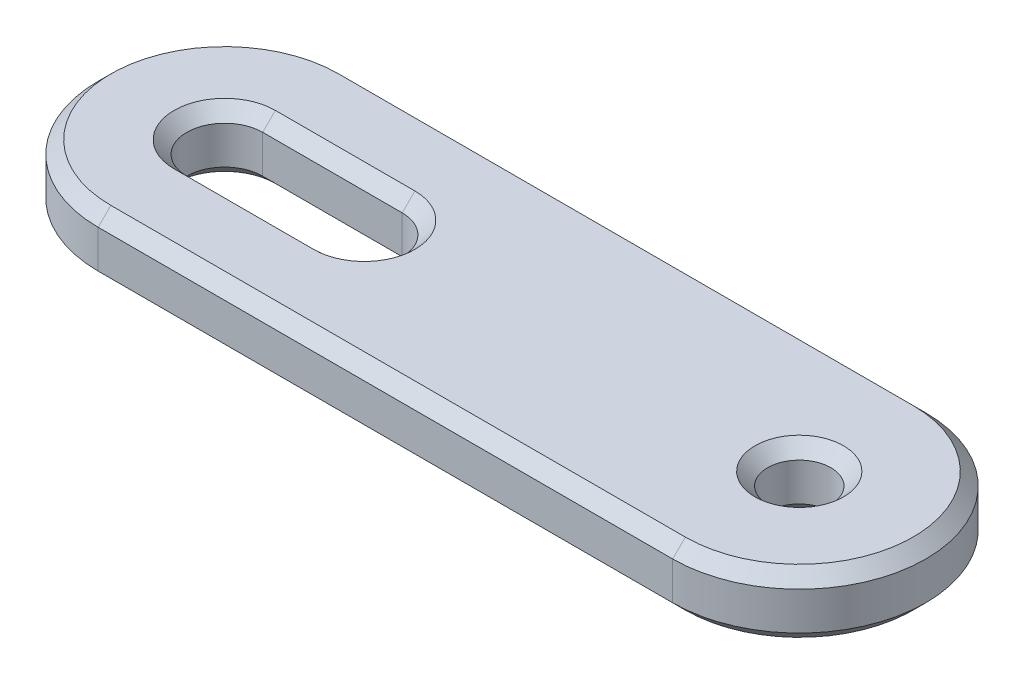
from build123d import *

# Parameters (mm, degrees)
SKETCH1_R           = 2.5
BOSS_EXTRUDE1_DEPTH = 5
CHAMFER1_SIZE       = 1


with BuildPart() as part:
    # Sketch1 → Boss-Extrude1 (new body)
    with BuildSketch(Plane(origin=(0, 0, 0), x_dir=(1, 0, 0), z_dir=(0, 1, 0))):
        with BuildLine():
            Line((0, -10), (-45.398085341, -10))
            ThreePointArc((-45.398085341, -10), (-55.398085341, 0), (-45.398085341, 10))
            Line((-45.398085341, 10), (0, 10))
            ThreePointArc((0, 10), (10, 0), (0, -10))
        make_face()
        with Locations(Location((0, 0, 0), (0, 0, 270))):
            Circle(SKETCH1_R, mode=Mode.SUBTRACT)
        with BuildLine():
            Line((-45.398085341, 3), (-34.372756479, 3))
            ThreePointArc((-34.372756479, 3), (-31.372756479, 0), (-34.372756479, -3))
            Line((-34.372756479, -3), (-45.398085341, -3))
            ThreePointArc((-45.398085341, -3), (-48.398085341, 0), (-45.398085341, 3))
        make_face(mode=Mode.SUBTRACT)
    extrude(amount=BOSS_EXTRUDE1_DEPTH)

    # Chamfer1
    chamfer1_edges = [part.edges().sort_by_distance(p)[0] for p in [
        (0, 0, -2.5),
        (0, 5, -2.5),
        (-55.398085341, 5, 0),
        (-22.69904267, 5, 10),
        (-48.398085341, 0, 0),
        (-39.88542091, 0, 3),
        (-31.372756479, 0, 0),
        (-39.88542091, 0, -3),
        (-48.398085341, 5, 0),
        (-39.88542091, 5, 3),
        (-31.372756479, 5, 0),
        (-39.88542091, 5, -3),
        (10, 5, 0),
        (-22.69904267, 0, 10),
        (-55.398085341, 0, 0),
        (-22.69904267, 0, -10),
        (10, 0, 0),
        (-22.69904267, 5, -10),
    ]]
    chamfer(chamfer1_edges, length=CHAMFER1_SIZE)


solid = part.part
